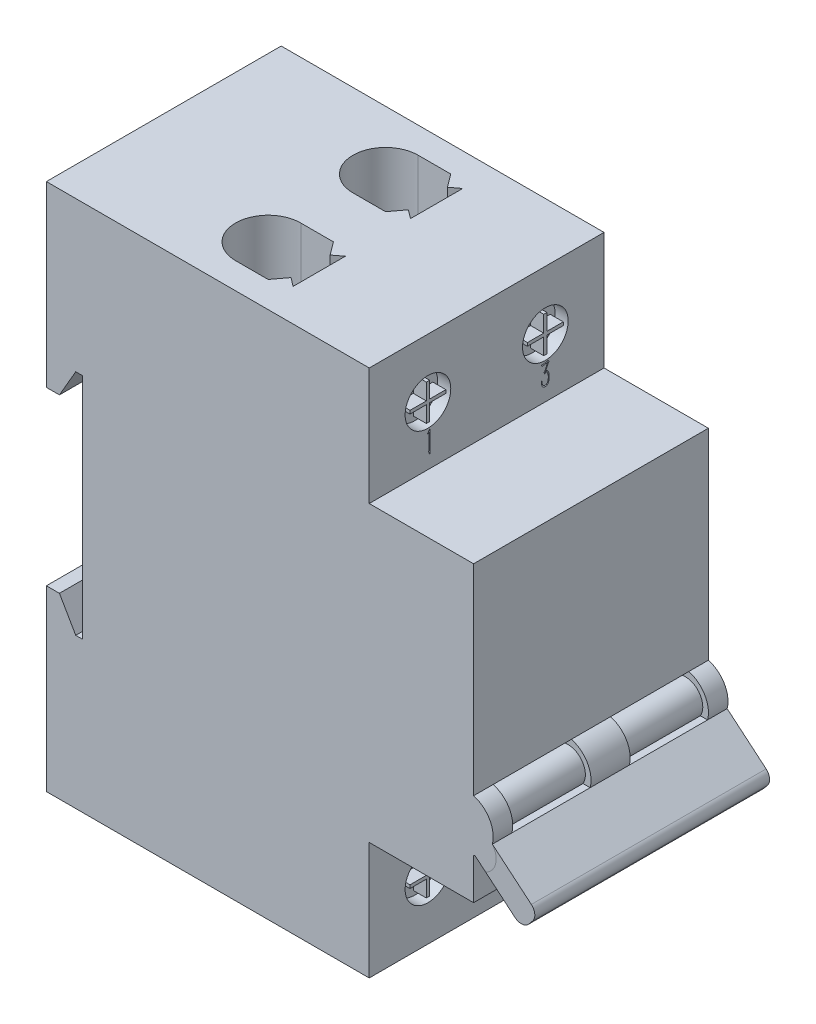
from build123d import *

# Parameters (mm, degrees)
BOSS_EXTRUDE1_DEPTH = 18
SKETCH2_R           = 3.5
CUT_EXTRUDE1_DEPTH  = 2
CUT_EXTRUDE5_DEPTH  = 15
SKETCH12_R          = 4.114641301
BOSS_EXTRUDE4_DEPTH = 18
BOSS_EXTRUDE5_DEPTH = 18
FILLET1_R           = 1.5
SKETCH15_W          = 12
SKETCH15_H          = 4.990244444
CUT_EXTRUDE9_DEPTH  = 5
BOSS_EXTRUDE6_REACH = 88.448
SKETCH16_R          = 2.68605677
LPATTERN2_COUNT     = 2
LPATTERN2_PITCH     = 18
CUT_EXTRUDE10_DEPTH = 1


with BuildPart() as part:
    # Sketch1 → Boss-Extrude1 (new body)
    with BuildSketch(Plane.XY):
        Polygon((0, 13.169872981), (2, 13.169872981), (4.5, 17.5), (5.5, 17.5), (5.5, -17.5), (4.5, -17.5), (2, -13.169872981), (0, -13.169872981), (0, -40.5), (49.5, -40.5), (49.5, -22.5), (65.5, -22.5), (65.5, 22.5), (49.5, 22.5), (49.5, 40.5), (0, 40.5), align=None)
    extrude(amount=-BOSS_EXTRUDE1_DEPTH)

    # Sketch2 → Cut-Extrude1 (cut)
    with BuildSketch(Plane(origin=(49.5, 0, 0), x_dir=(0, 0, -1), z_dir=(1, 0, 0))):
        with Locations((9, 31.5)):
            Circle(SKETCH2_R)
        Polygon((8.75, 34.25), (9.25, 34.25), (9.25, 31.75), (11.75, 31.75), (11.75, 31.25), (9.25, 31.25), (9.25, 28.75), (8.75, 28.75), (8.75, 31.25), (6.25, 31.25), (6.25, 31.75), (8.75, 31.75), align=None, mode=Mode.SUBTRACT)
    cut_extrude1 = extrude(amount=-CUT_EXTRUDE1_DEPTH, mode=Mode.SUBTRACT)

    # Sketch11 → Cut-Extrude5 (cut)
    with BuildSketch(Plane(origin=(0, 40.5, 0), x_dir=(1, 0, 0), z_dir=(0, 1, 0))):
        with BuildLine():
            Line((32.833333333, 5), (32.833333333, 13))
            Line((32.833333333, 13), (31.5, 12))
            Line((31.5, 12), (30, 14))
            Line((30, 14), (25, 14))
            ThreePointArc((25, 14), (21.464466094, 12.535533906), (20, 9))
            ThreePointArc((20, 9), (21.464466094, 5.464466094), (25, 4))
            Line((25, 4), (30, 4))
            Line((30, 4), (31.5, 6))
            Line((31.5, 6), (32.833333333, 5))
        make_face()
    cut_extrude5 = extrude(amount=-CUT_EXTRUDE5_DEPTH, mode=Mode.SUBTRACT)

    # Mirror1: Cut-Extrude1, Cut-Extrude5 across plane
    add(cut_extrude1.mirror(Plane.ZX), mode=Mode.SUBTRACT)
    add(cut_extrude5.mirror(Plane.ZX), mode=Mode.SUBTRACT)

    # Sketch12 → Boss-Extrude4 (add, through all)
    with BuildSketch(Plane.XY):
        with Locations((64.39025967, -12.26560275)):
            Circle(SKETCH12_R)
    extrude(amount=-BOSS_EXTRUDE4_DEPTH)

    # Sketch13 → Boss-Extrude5 (add, through all)
    with BuildSketch(Plane.XY):
        Polygon((65.5, -10.881779635), (75.5, -19.272775947), (72.999147741, -22.253175611), (65.5, -15.960643508), align=None)
    extrude(amount=-BOSS_EXTRUDE5_DEPTH)

    # Fillet1
    fillet1_edges = [part.edges().sort_by_distance(p)[0] for p in [
        (75.5, -19.272775947, -9),
        (72.999147741, -22.253175611, -9),
    ]]
    fillet(fillet1_edges, radius=FILLET1_R)

    # Sketch15 → Cut-Extrude9 (cut, symmetric)
    with BuildSketch(Plane(origin=(65.5, 0, 0), x_dir=(0, 0, -1), z_dir=(1, 0, 0))):
        with Locations((9, -10.798560231)):
            Rectangle(SKETCH15_W, SKETCH15_H)
    extrude(amount=CUT_EXTRUDE9_DEPTH, both=True, mode=Mode.SUBTRACT)

    # Sketch16 → Boss-Extrude6 (add, up to next)
    with BuildSketch(Plane.XY.offset(-15), mode=Mode.PRIVATE) as boss_extrude6_sk1:
        with Locations((64.953909061, -11.94282373)):
            Circle(SKETCH16_R)
    boss_extrude6_tool1 = extrude(boss_extrude6_sk1.sketch, amount=BOSS_EXTRUDE6_REACH, mode=Mode.PRIVATE) - part.part
    add(boss_extrude6_tool1.solids().sort_by_distance((64.953909, -11.942824, -15))[0])


with BuildPart() as lpattern2_1:
    # LPattern2: pattern copy
    add(part.part.moved(Location(Vector(0, 0, -1) * (1 * LPATTERN2_PITCH))))


with BuildPart() as part_1:
    add(part.part)

    # Combine1: union LPattern2_1
    add(lpattern2_1.part)

    # Sketch19 → Cut-Extrude10 (cut)
    # profile 1 of 4: a face of its own
    with BuildSketch(Plane(origin=(49.5, 0, 0), x_dir=(0, 0, -1), z_dir=(1, 0, 0))):
        with BuildLine():
            Line((9.268616193, 27.777022397), (9.323804772, 27.777022397))
            Line((9.323804772, 27.777022397), (9.31858423, 25.103359495))
            add(Edge.make_bspline(
                [(9.31858423, 25.103359495), (9.317989513, 25.079247206), (9.316849208, 25.033014576), (9.316756663, 24.966867672), (9.314581251, 24.906977786), (9.31440798, 24.853259172), (9.312790378, 24.805782007), (9.310919778, 24.764536358), (9.310742036, 24.729444909), (9.307433278, 24.674522263), (9.303490456, 24.59900772), (9.293712461, 24.521229024), (9.285928441, 24.465808449), (9.278015344, 24.440580035), (9.267990261, 24.420618486), (9.257985248, 24.422946371), (9.253700361, 24.423943344)],
                knots=[0, 0, 0, 0, 1.45038606, 2.780953852, 3.977268029, 5.053718292, 6.010937745, 6.833690271, 7.536464333, 8.120251454, 10.142880859, 12.069479857, 12.873132744, 13.440417135, 13.76034519, 14, 14, 14, 14], degree=3))
            add(Edge.make_bspline(
                [(9.253700361, 24.423943344), (9.252709832, 24.424693106), (9.248470125, 24.427902274), (9.238359598, 24.434694901), (9.226346206, 24.452902941), (9.221087494, 24.469237998), (9.217902364, 24.479131922)],
                knots=[0, 0, 0, 0, 0.221265066, 0.947068446, 2.150880552, 4, 4, 4, 4], degree=3))
            Line((9.217902364, 24.479131922), (9.193291241, 24.544761583))
            Line((9.193291241, 24.544761583), (9.13735687, 24.725988943))
            add(Edge.make_bspline(
                [(9.13735687, 24.725988943), (9.130623579, 24.743040571), (9.118894532, 24.772743625), (9.107062513, 24.811822119), (9.098086344, 24.836775388), (9.09570055, 24.857001098), (9.107192928, 24.875972867), (9.11565667, 24.905183607), (9.128680107, 24.942469195), (9.140978693, 24.986476292), (9.151841244, 25.034025265), (9.161626509, 25.085400436), (9.167172099, 25.143283169), (9.169892428, 25.198549028), (9.171980118, 25.251758462), (9.172359418, 25.302984326), (9.173405582, 25.363637315), (9.173242151, 25.407393199), (9.173154868, 25.43076201)],
                knots=[0, 0, 0, 0, 1.220359697, 2.125803599, 2.712350858, 2.994193817, 3.439826662, 4.12562012, 5.031064022, 6.063176816, 7.167225426, 8.277459231, 9.542238136, 11.034069985, 11.961482632, 13.08703073, 14.444263491, 16, 16, 16, 16], degree=3))
            Line((9.173154868, 25.43076201), (9.177629617, 27.404126595))
            Line((9.177629617, 27.404126595), (8.915856764, 27.177405947))
            Line((8.915856764, 27.177405947), (8.895720391, 27.263171982))
            add(Edge.make_bspline(
                [(8.895720391, 27.263171982), (8.916998829, 27.285159101), (8.956886141, 27.326374863), (9.010193269, 27.385718152), (9.054036517, 27.437218727), (9.099702186, 27.497425312), (9.150830111, 27.572352034), (9.188586471, 27.633910013), (9.208207073, 27.665899448)],
                knots=[0, 0, 0, 0, 1.077185482, 2.019228619, 2.808185376, 3.45765616, 4.678836699, 6, 6, 6, 6], degree=3))
            Line((9.208207073, 27.665899448), (9.268616193, 27.777022397))
        make_face()
    # profile 2 of 4: a face of its own
    with BuildSketch(Plane(origin=(49.5, 0, 0), x_dir=(0, 0, -1), z_dir=(1, 0, 0))):
        with BuildLine():
            add(Edge.make_bspline(
                [(26.894587034, 26.553178374), (26.905758668, 26.576305419), (26.92727936, 26.620856647), (26.95866931, 26.685209589), (26.987953271, 26.744293665), (27.012999895, 26.799120123), (27.036354733, 26.848480227), (27.057155241, 26.892902394), (27.075128281, 26.932401147), (27.094050096, 26.976253222), (27.113674908, 27.02200111), (27.132673375, 27.066809999), (27.146489283, 27.098818021), (27.153632136, 27.115750937), (27.156359887, 27.122217369)],
                knots=[0, 0, 0, 0, 1.475873638, 2.843077615, 4.114458223, 5.26483622, 6.306479236, 7.252326145, 8.083448402, 8.799989154, 9.996708352, 10.943956596, 11.596712522, 12, 12, 12, 12], degree=3))
            Line((27.156359887, 27.122217369), (27.317450874, 27.55030175))
            add(Edge.make_bspline(
                [(27.317450874, 27.55030175), (27.282414717, 27.546873059), (27.20596755, 27.539391824), (27.108407493, 27.533451709), (27.027289802, 27.529125888), (26.971629196, 27.524461766), (26.922889389, 27.520102343), (26.892842398, 27.516785719), (26.87892541, 27.515249544)],
                knots=[0, 0, 0, 0, 1.440114021, 3.142257811, 3.998086789, 4.76330671, 5.427195687, 6, 6, 6, 6], degree=3))
            Line((26.87892541, 27.515249544), (26.728275506, 27.48989263))
            add(Edge.make_bspline(
                [(26.728275506, 27.48989263), (26.721544061, 27.488477454), (26.70317884, 27.484616469), (26.669215876, 27.474073313), (26.620302936, 27.461107664), (26.58307352, 27.450445131), (26.561963978, 27.444399342)],
                knots=[0, 0, 0, 0, 0.478461291, 1.305373098, 2.472113022, 4, 4, 4, 4], degree=3))
            Line((26.561963978, 27.444399342), (26.511995941, 27.424262968))
            Line((26.511995941, 27.424262968), (26.38595716, 27.61071087))
            add(Edge.make_bspline(
                [(26.38595716, 27.61071087), (26.380634962, 27.618010698), (26.371549402, 27.630472284), (26.364006769, 27.647807605), (26.358407972, 27.65985087), (26.363426008, 27.671978454), (26.383268796, 27.670159902), (26.398250403, 27.659523203), (26.417386103, 27.649289333), (26.439402155, 27.647850003), (26.466093406, 27.646283592), (26.485655754, 27.64932396), (26.496334317, 27.650983616)],
                knots=[0, 0, 0, 0, 1.323589942, 2.259509366, 2.829398404, 3.190947808, 3.965341466, 5.19662492, 6.050472624, 7.088782, 8.410843841, 10, 10, 10, 10], degree=3))
            Line((26.496334317, 27.650983616), (26.657425304, 27.656204158))
            Line((26.657425304, 27.656204158), (27.292093959, 27.73152911))
            Line((27.292093959, 27.73152911), (27.342061997, 27.777022397))
            Line((27.342061997, 27.777022397), (27.382334743, 27.817295144))
            add(Edge.make_bspline(
                [(27.382334743, 27.817295144), (27.383583719, 27.815808411), (27.388703828, 27.809713632), (27.399726504, 27.795210802), (27.419326367, 27.771910062), (27.434144734, 27.752492469), (27.442743863, 27.7412244)],
                knots=[0, 0, 0, 0, 0.23984028, 0.983211964, 2.249351781, 4, 4, 4, 4], degree=3))
            Line((27.442743863, 27.7412244), (27.53895098, 27.62040616))
            add(Edge.make_bspline(
                [(27.53895098, 27.62040616), (27.54541144, 27.612018118), (27.556147701, 27.598078521), (27.564112726, 27.575785092), (27.555951012, 27.56068078), (27.544549588, 27.547733644), (27.52606782, 27.532183142), (27.511424617, 27.521362113), (27.503152983, 27.515249544)],
                knots=[0, 0, 0, 0, 1.419029252, 2.358201718, 2.827787952, 3.596253847, 4.642174893, 6, 6, 6, 6], degree=3))
            Line((27.503152983, 27.515249544), (27.447964405, 27.469756256))
            add(Edge.make_bspline(
                [(27.447964405, 27.469756256), (27.43183587, 27.429222959), (27.401234241, 27.352316717), (27.357143356, 27.242865851), (27.316798395, 27.145548297), (27.281372724, 27.059514144), (27.248833746, 26.985741252), (27.221970898, 26.923143149), (27.197785591, 26.872921774), (27.182992591, 26.843523203), (27.176496261, 26.830612851)],
                knots=[0, 0, 0, 0, 1.507300768, 2.859891598, 4.076963614, 5.147345159, 6.074452096, 6.862861548, 7.500626815, 8, 8, 8, 8], degree=3))
            Line((27.176496261, 26.830612851), (27.025100565, 26.543483084))
            add(Edge.make_bspline(
                [(27.025100565, 26.543483084), (27.042996023, 26.54491193), (27.077268983, 26.547648422), (27.129573753, 26.552872254), (27.186562807, 26.54568692), (27.236547135, 26.525696313), (27.279075075, 26.501029434), (27.313152721, 26.476392071), (27.345708772, 26.444370394), (27.378905936, 26.406726573), (27.412180649, 26.361796719), (27.442768582, 26.307377441), (27.474610228, 26.245235491), (27.514431877, 26.150532156), (27.557460863, 26.023817162), (27.583604576, 25.86466242), (27.596521571, 25.705205737), (27.598417879, 25.599087053), (27.5993601, 25.546359708)],
                knots=[0, 0, 0, 0, 0.660541429, 1.265053373, 1.928435853, 2.750244091, 3.225390118, 3.735570922, 4.291687282, 4.900607759, 5.580848831, 6.342918567, 7.193367346, 8.147740655, 10.119512469, 12.097611575, 14.061014616, 16, 16, 16, 16], degree=3))
            add(Edge.make_bspline(
                [(27.5993601, 25.546359708), (27.597369738, 25.505079829), (27.593588689, 25.426661312), (27.584450789, 25.315849931), (27.570814377, 25.218634004), (27.550955275, 25.109031476), (27.515932295, 24.987942252), (27.472665848, 24.876226259), (27.431585008, 24.795741244), (27.396962993, 24.742372127), (27.359042011, 24.69462663), (27.318290969, 24.652844146), (27.275901478, 24.618507711), (27.234760539, 24.588977252), (27.193130085, 24.568106084), (27.139235736, 24.550670286), (27.073375552, 24.538651683), (27.020920749, 24.536243809), (26.995268901, 24.535066293)],
                knots=[0, 0, 0, 0, 1.512752116, 2.8737433, 4.067977017, 5.104892351, 6.948544146, 8.672095895, 9.482011449, 10.251829035, 10.996496654, 11.710742831, 12.38300564, 12.991319199, 13.561044299, 14.079002633, 15.060579187, 16, 16, 16, 16], degree=3))
            add(Edge.make_bspline(
                [(26.995268901, 24.535066293), (26.973388966, 24.534693339), (26.93129448, 24.53397582), (26.870237534, 24.538946321), (26.81462808, 24.55032289), (26.762475647, 24.565798969), (26.713633203, 24.590272598), (26.666979223, 24.625233083), (26.620013623, 24.668282899), (26.574983014, 24.721112889), (26.533770386, 24.781638563), (26.497735149, 24.848588226), (26.46779483, 24.921014069), (26.438030374, 25.024086001), (26.412802475, 25.155884677), (26.408308057, 25.262588435), (26.406093533, 25.315164311)],
                knots=[0, 0, 0, 0, 0.828828519, 1.594571005, 2.314948186, 2.97625877, 3.650192192, 4.371738268, 5.178272596, 6.059897072, 6.995131469, 7.947518938, 8.935744196, 9.957858231, 12.008325587, 14, 14, 14, 14], degree=3))
            Line((26.406093533, 25.315164311), (26.400872992, 25.511307503))
            Line((26.400872992, 25.511307503), (26.456061571, 25.511307503))
            add(Edge.make_bspline(
                [(26.456061571, 25.511307503), (26.460281768, 25.482221028), (26.468363821, 25.426517849), (26.480120095, 25.346152318), (26.492296408, 25.272893692), (26.50601877, 25.186199105), (26.528872927, 25.088850434), (26.567375212, 24.984077852), (26.619589704, 24.89555163), (26.680895946, 24.822599949), (26.752597249, 24.769647856), (26.829354682, 24.736246775), (26.90758436, 24.720476219), (26.959416586, 24.720672281), (26.984827818, 24.720768402)],
                knots=[0, 0, 0, 0, 0.994021113, 1.903638599, 2.746793397, 3.505624798, 4.871908371, 6.122639036, 7.264652637, 8.331625701, 9.323760524, 10.250011688, 11.142051883, 12, 12, 12, 12], degree=3))
            add(Edge.make_bspline(
                [(26.984827818, 24.720768402), (27.005270774, 24.722531252), (27.045310018, 24.725983941), (27.103371268, 24.739128694), (27.157066245, 24.761557691), (27.207260378, 24.790239493), (27.252440104, 24.827641551), (27.293102101, 24.871713388), (27.327537611, 24.924069674), (27.366130118, 25.004224122), (27.403636112, 25.114727617), (27.431856393, 25.255086396), (27.450219792, 25.398256076), (27.458846817, 25.540709206), (27.460022294, 25.681050273), (27.448482407, 25.772899132), (27.442743863, 25.818573644)],
                knots=[0, 0, 0, 0, 0.647840119, 1.268849254, 1.871153999, 2.479976942, 3.088343857, 3.716462885, 4.367721208, 5.059616847, 6.52246665, 8.039623249, 9.575767262, 11.078710543, 12.547304005, 14, 14, 14, 14], degree=3))
            add(Edge.make_bspline(
                [(27.442743863, 25.818573644), (27.434719682, 25.867804036), (27.418857721, 25.965121191), (27.382165945, 26.081930294), (27.346034778, 26.169154367), (27.313799504, 26.227674778), (27.277262229, 26.279947351), (27.235874793, 26.32378913), (27.193919543, 26.35976614), (27.15180766, 26.383772702), (27.110219955, 26.396125961), (27.083571503, 26.393410031), (27.070593853, 26.392087388)],
                knots=[0, 0, 0, 0, 2.019199264, 3.991492233, 4.943861116, 5.841091039, 6.693606335, 7.520378909, 8.278781735, 8.923571305, 9.475785111, 10, 10, 10, 10], degree=3))
            Line((27.070593853, 26.392087388), (26.990048359, 26.382392097))
            Line((26.990048359, 26.382392097), (26.954996154, 26.316762436))
            add(Edge.make_bspline(
                [(26.954996154, 26.316762436), (26.950317629, 26.308583345), (26.94216181, 26.294325183), (26.931016972, 26.275479105), (26.922115728, 26.264440522), (26.915359483, 26.254924454), (26.905592767, 26.258125672), (26.899310799, 26.269064642), (26.889268494, 26.285168339), (26.882736067, 26.298999064), (26.87892541, 26.307067145)],
                knots=[0, 0, 0, 0, 1.659028505, 2.892093886, 3.763458346, 4.288089223, 4.647361994, 5.327919393, 6.441255868, 8, 8, 8, 8], degree=3))
            Line((26.87892541, 26.307067145), (26.798379917, 26.46293759))
            add(Edge.make_bspline(
                [(26.798379917, 26.46293759), (26.792557932, 26.471896017), (26.782408552, 26.48751311), (26.786808583, 26.505315301), (26.788684626, 26.512905628)],
                knots=[0, 0, 0, 0, 1.147259222, 2, 2, 2, 2], degree=3))
            Line((26.788684626, 26.512905628), (26.828957373, 26.528567251))
            Line((26.828957373, 26.528567251), (26.894587034, 26.553178374))
        make_face()
    # profile 3 of 4: a face of its own
    with BuildSketch(Plane(origin=(49.5, 0, 0), x_dir=(0, 0, -1), z_dir=(1, 0, 0))):
        with BuildLine():
            Line((8.730154654, -24.847385713), (8.654083911, -24.847385713))
            add(Edge.make_bspline(
                [(8.654083911, -24.847385713), (8.652516507, -24.823276458), (8.649528375, -24.777314072), (8.646445032, -24.711674798), (8.64514292, -24.652738754), (8.643838503, -24.580888811), (8.645850242, -24.490276951), (8.65125193, -24.417292602), (8.654083911, -24.379028585)],
                knots=[0, 0, 0, 0, 0.927540379, 1.768282303, 2.522502339, 3.190652681, 4.527123766, 6, 6, 6, 6], degree=3))
            add(Edge.make_bspline(
                [(8.654083911, -24.379028585), (8.656043818, -24.350662308), (8.659834054, -24.295805178), (8.669837058, -24.216742672), (8.681413565, -24.143478296), (8.69646412, -24.074567742), (8.7167999, -24.007131882), (8.745750083, -23.939303027), (8.781856415, -23.868757962), (8.824515086, -23.797966017), (8.871321724, -23.731168134), (8.923860232, -23.676810886), (8.978846052, -23.635379689), (9.03734966, -23.610721813), (9.093521598, -23.595388131), (9.144745804, -23.583326557), (9.190777383, -23.574897147), (9.219860114, -23.573997547), (9.233563987, -23.573573652)],
                knots=[0, 0, 0, 0, 1.238521709, 2.395159043, 3.470603583, 4.46912877, 5.466066804, 6.534123646, 7.677244524, 8.916145015, 10.13365226, 11.221244199, 12.198275335, 13.109907183, 13.966820176, 14.733954848, 15.403435577, 16, 16, 16, 16], degree=3))
            add(Edge.make_bspline(
                [(9.233563987, -23.573573652), (9.251028183, -23.574861334), (9.285536892, -23.577405754), (9.336298249, -23.589194749), (9.3853233, -23.606192719), (9.448027995, -23.63647274), (9.521351042, -23.683947637), (9.583729421, -23.746290041), (9.626893488, -23.803356357), (9.65729834, -23.851924205), (9.684241838, -23.90615696), (9.718077941, -23.984958998), (9.75347521, -24.089530022), (9.779001912, -24.221603947), (9.795369003, -24.35875684), (9.802857469, -24.498968402), (9.804249869, -24.637798018), (9.796098136, -24.728340443), (9.792161899, -24.772060761)],
                knots=[0, 0, 0, 0, 0.570779476, 1.127842599, 1.694919432, 2.261066821, 3.397481896, 4.527710891, 5.118384485, 5.730727279, 6.394748858, 7.092559246, 8.529363642, 9.986910621, 11.474321506, 13.03467297, 14.568129345, 16, 16, 16, 16], degree=3))
            add(Edge.make_bspline(
                [(9.792161899, -24.772060761), (9.784182525, -24.817033009), (9.768104722, -24.907648497), (9.733475036, -25.016748296), (9.701178927, -25.099692259), (9.674177686, -25.155273163), (9.645327126, -25.204477751), (9.603609389, -25.262667052), (9.539900956, -25.328718412), (9.480864698, -25.373013219), (9.449843553, -25.396288334)],
                knots=[0, 0, 0, 0, 1.490916612, 3.004077927, 3.729534125, 4.397912905, 5.020560084, 5.590839424, 6.734084393, 8, 8, 8, 8], degree=3))
            Line((9.449843553, -25.396288334), (9.202986532, -25.552158779))
            add(Edge.make_bspline(
                [(9.202986532, -25.552158779), (9.171529528, -25.573514544), (9.111881044, -25.614009149), (9.032233852, -25.680155183), (8.965383351, -25.749851267), (8.914854257, -25.826914516), (8.875609345, -25.906240314), (8.840761113, -25.985891172), (8.814452469, -26.073684748), (8.795740738, -26.152376603), (8.782979957, -26.218465922), (8.776587827, -26.264558022), (8.771395086, -26.305294785), (8.770736473, -26.330751604), (8.770427401, -26.34269788)],
                knots=[0, 0, 0, 0, 1.453572249, 2.75625039, 3.953730064, 5.132566341, 6.263730064, 7.337486329, 8.453238547, 9.76321854, 10.430854957, 11.026567013, 11.543191201, 12, 12, 12, 12], degree=3))
            Line((8.770427401, -26.34269788), (8.759986319, -26.553756904))
            Line((8.759986319, -26.553756904), (9.660902577, -26.52392524))
            add(Edge.make_bspline(
                [(9.660902577, -26.52392524), (9.672462855, -26.523278875), (9.692767296, -26.522143602), (9.71228111, -26.500870216), (9.71662466, -26.474895395), (9.724332018, -26.442947113), (9.730061911, -26.397152102), (9.734482123, -26.362325748), (9.736973321, -26.34269788)],
                knots=[0, 0, 0, 0, 0.925905201, 1.626257371, 2.181371879, 3.087088273, 4.358305093, 6, 6, 6, 6], degree=3))
            Line((9.736973321, -26.34269788), (9.757109694, -25.904172416))
            Line((9.757109694, -25.904172416), (9.827214105, -25.904172416))
            Line((9.827214105, -25.904172416), (9.852571019, -26.568672736))
            add(Edge.make_bspline(
                [(9.852571019, -26.568672736), (9.853418715, -26.581591346), (9.854901335, -26.604186009), (9.855623054, -26.634075483), (9.855643482, -26.654888005), (9.855328713, -26.671692005), (9.849916523, -26.68638406), (9.84488751, -26.703431679), (9.825269802, -26.713062781), (9.797070739, -26.716144309), (9.754214435, -26.720508585), (9.720578586, -26.720229453), (9.701175324, -26.720068432)],
                knots=[0, 0, 0, 0, 1.385018147, 2.4223982, 3.193529914, 3.619812046, 4.200562765, 4.878496499, 5.402948042, 6.404258339, 7.925751149, 10, 10, 10, 10], degree=3))
            Line((9.701175324, -26.720068432), (8.699577199, -26.745425346))
            add(Edge.make_bspline(
                [(8.699577199, -26.745425346), (8.687401759, -26.745460965), (8.663403069, -26.745531172), (8.638810076, -26.721667198), (8.628486444, -26.692453054), (8.623319507, -26.658091359), (8.61985857, -26.612504766), (8.618196149, -26.534098628), (8.621750352, -26.422538741), (8.629756092, -26.330484316), (8.633947537, -26.28228876)],
                knots=[0, 0, 0, 0, 0.556373901, 1.096654043, 1.476064089, 2.012759395, 2.73145082, 3.635924119, 5.715166189, 8, 8, 8, 8], degree=3))
            add(Edge.make_bspline(
                [(8.633947537, -26.28228876), (8.637667097, -26.254157079), (8.644832261, -26.199965695), (8.659400716, -26.121959966), (8.674933052, -26.049553187), (8.691789735, -25.982789164), (8.710398684, -25.922019627), (8.7307103, -25.867314144), (8.751766421, -25.81779166), (8.783393806, -25.761768771), (8.82358975, -25.700701936), (8.86931043, -25.634857188), (8.91333054, -25.579003158), (8.970866969, -25.517554724), (9.048760279, -25.450483145), (9.114195614, -25.401371673), (9.147797953, -25.37615196)],
                knots=[0, 0, 0, 0, 1.103491021, 2.125706759, 3.085324024, 3.98349739, 4.803138144, 5.555704107, 6.252741852, 6.89323317, 8.054555834, 9.09539633, 10.010480884, 10.817709087, 12.365830683, 14, 14, 14, 14], degree=3))
            Line((9.147797953, -25.37615196), (9.354382227, -25.244892638))
            add(Edge.make_bspline(
                [(9.354382227, -25.244892638), (9.370921509, -25.233896319), (9.402660187, -25.212794517), (9.446498042, -25.179198736), (9.483871457, -25.144340724), (9.516078649, -25.106724377), (9.545234203, -25.063196929), (9.569178512, -25.008940647), (9.59449199, -24.945031971), (9.624006101, -24.845602012), (9.654437281, -24.714363208), (9.666102897, -24.552212497), (9.65987102, -24.387958902), (9.640818996, -24.278938888), (9.631070913, -24.22315814)],
                knots=[0, 0, 0, 0, 0.635613896, 1.219735276, 1.765761318, 2.268061313, 2.802129131, 3.435697723, 4.161225462, 5.001884758, 6.75303811, 8.46119913, 10.189351173, 12, 12, 12, 12], degree=3))
            add(Edge.make_bspline(
                [(9.631070913, -24.22315814), (9.623725567, -24.194721139), (9.609399703, -24.139259545), (9.582284963, -24.059364957), (9.547186593, -23.986598886), (9.509619076, -23.918624202), (9.462554079, -23.859122868), (9.399862794, -23.816389074), (9.325801546, -23.787822518), (9.27162761, -23.782792113), (9.243259278, -23.780157927)],
                knots=[0, 0, 0, 0, 1.101106684, 2.147523679, 3.156537618, 4.125318695, 5.058520457, 5.968677808, 6.93629249, 8, 8, 8, 8], degree=3))
            add(Edge.make_bspline(
                [(9.243259278, -23.780157927), (9.228326882, -23.78000505), (9.198543172, -23.779700127), (9.15418165, -23.786427429), (9.111033958, -23.800532746), (9.054355541, -23.826097853), (8.988862492, -23.873718727), (8.91992613, -23.945569602), (8.863064593, -24.033301084), (8.819285565, -24.13496587), (8.786366995, -24.250789776), (8.759643561, -24.380596909), (8.742096183, -24.52603338), (8.737193746, -24.627827981), (8.734629404, -24.681074185)],
                knots=[0, 0, 0, 0, 0.469335518, 0.936122588, 1.403629858, 1.893624907, 2.887406355, 3.927357629, 5.011993806, 6.157121359, 7.396943717, 8.794309501, 10.323183677, 12, 12, 12, 12], degree=3))
            Line((8.734629404, -24.681074185), (8.730154654, -24.847385713))
        make_face()
    # profile 4 of 4: a face of its own
    with BuildSketch(Plane(origin=(49.5, 0, 0), x_dir=(0, 0, -1), z_dir=(1, 0, 0))):
        with BuildLine():
            Line((27.186191551, -25.808711091), (26.476197944, -25.848983838))
            Line((26.476197944, -25.848983838), (26.426229906, -25.92430879))
            add(Edge.make_bspline(
                [(26.426229906, -25.92430879), (26.422969209, -25.932202289), (26.418041285, -25.944131812), (26.399821496, -25.956434612), (26.386153034, -25.938787294), (26.379694111, -25.927278587), (26.375516077, -25.91983404)],
                knots=[0, 0, 0, 0, 1.282902353, 1.938863145, 2.666728425, 4, 4, 4, 4], degree=3))
            Line((26.375516077, -25.91983404), (26.280054752, -25.728165598))
            add(Edge.make_bspline(
                [(26.280054752, -25.728165598), (26.275970963, -25.716847246), (26.269236836, -25.698183401), (26.264334142, -25.673131982), (26.265728107, -25.655463636), (26.268963559, -25.646337108), (26.270359461, -25.642399563)],
                knots=[0, 0, 0, 0, 1.63130738, 2.690008936, 3.434818089, 4, 4, 4, 4], degree=3))
            Line((26.270359461, -25.642399563), (26.310632208, -25.632704272))
            Line((26.310632208, -25.632704272), (26.365820786, -25.602126817))
            Line((26.365820786, -25.602126817), (27.216769007, -23.548216738))
            Line((27.216769007, -23.548216738), (27.327146165, -23.548216738))
            Line((27.327146165, -23.548216738), (27.327146165, -25.62226319))
            add(Edge.make_bspline(
                [(27.327146165, -25.62226319), (27.337517711, -25.622341822), (27.355153283, -25.622475527), (27.371235704, -25.615458278), (27.377859994, -25.612567899)],
                knots=[0, 0, 0, 0, 1.176207474, 2, 2, 2, 2], degree=3))
            Line((27.377859994, -25.612567899), (27.453184946, -25.581990443))
            add(Edge.make_bspline(
                [(27.453184946, -25.581990443), (27.462922591, -25.578356102), (27.480279634, -25.571878005), (27.502629071, -25.562149087), (27.518450332, -25.554658262), (27.525822287, -25.549000794), (27.528509898, -25.546938238)],
                knots=[0, 0, 0, 0, 1.495147538, 2.665053038, 3.513315187, 4, 4, 4, 4], degree=3))
            Line((27.528509898, -25.546938238), (27.563562103, -25.517106574))
            Line((27.563562103, -25.517106574), (27.704516717, -25.662535937))
            add(Edge.make_bspline(
                [(27.704516717, -25.662535937), (27.711697463, -25.671177462), (27.723452054, -25.685323286), (27.728582435, -25.70926226), (27.723689862, -25.725451473), (27.714543829, -25.737110002), (27.698601358, -25.741996953), (27.686866477, -25.742677653), (27.679905594, -25.74308143)],
                knots=[0, 0, 0, 0, 1.690587597, 2.767423091, 3.557953073, 4.202677464, 4.933866242, 6, 6, 6, 6], degree=3))
            Line((27.679905594, -25.74308143), (27.327146165, -25.783354176))
            Line((27.327146165, -25.783354176), (27.327146165, -26.685016226))
            add(Edge.make_bspline(
                [(27.327146165, -26.685016226), (27.327128212, -26.687751147), (27.327067793, -26.696955205), (27.328226229, -26.716330922), (27.328695969, -26.747160979), (27.329300443, -26.7854712), (27.330335667, -26.823912608), (27.330001199, -26.855048118), (27.327983039, -26.874682486), (27.323236362, -26.887300824), (27.313944894, -26.889560225), (27.309175758, -26.887373218), (27.307009791, -26.88637996)],
                knots=[0, 0, 0, 0, 0.375701713, 1.264380521, 2.665139726, 4.612257271, 6.525225464, 7.960129458, 8.858599367, 9.286556546, 9.675980055, 10, 10, 10, 10], degree=3))
            add(Edge.make_bspline(
                [(27.307009791, -26.88637996), (27.302798935, -26.883877082), (27.290105158, -26.876332067), (27.278979998, -26.851983484), (27.265612394, -26.826711093), (27.259603022, -26.808412858), (27.257041754, -26.800613925)],
                knots=[0, 0, 0, 0, 0.572299195, 1.725216547, 3.030459198, 4, 4, 4, 4], degree=3))
            Line((27.257041754, -26.800613925), (27.211548466, -26.709627349))
            Line((27.211548466, -26.709627349), (27.186191551, -26.639522938))
            add(Edge.make_bspline(
                [(27.186191551, -26.639522938), (27.182335483, -26.631121959), (27.175357852, -26.615920221), (27.167714287, -26.594965646), (27.160889762, -26.579495575), (27.157090728, -26.561090907), (27.161547109, -26.532339541), (27.171368715, -26.492075887), (27.183163945, -26.449032995), (27.188705787, -26.409701413), (27.190980879, -26.375794404), (27.191266296, -26.353888053), (27.191412093, -26.34269788)],
                knots=[0, 0, 0, 0, 0.908031708, 1.643101311, 2.192199313, 2.565975908, 3.473020803, 5.002279505, 6.661670863, 7.846934984, 8.900174221, 10, 10, 10, 10], degree=3))
            Line((27.191412093, -26.34269788), (27.186191551, -25.808711091))
        make_face()
        Polygon((27.191412093, -25.642399563), (27.191412093, -23.971080578), (26.481418485, -25.67819756), align=None, mode=Mode.SUBTRACT)
    extrude(amount=-CUT_EXTRUDE10_DEPTH, mode=Mode.SUBTRACT)


solid = part_1.part
